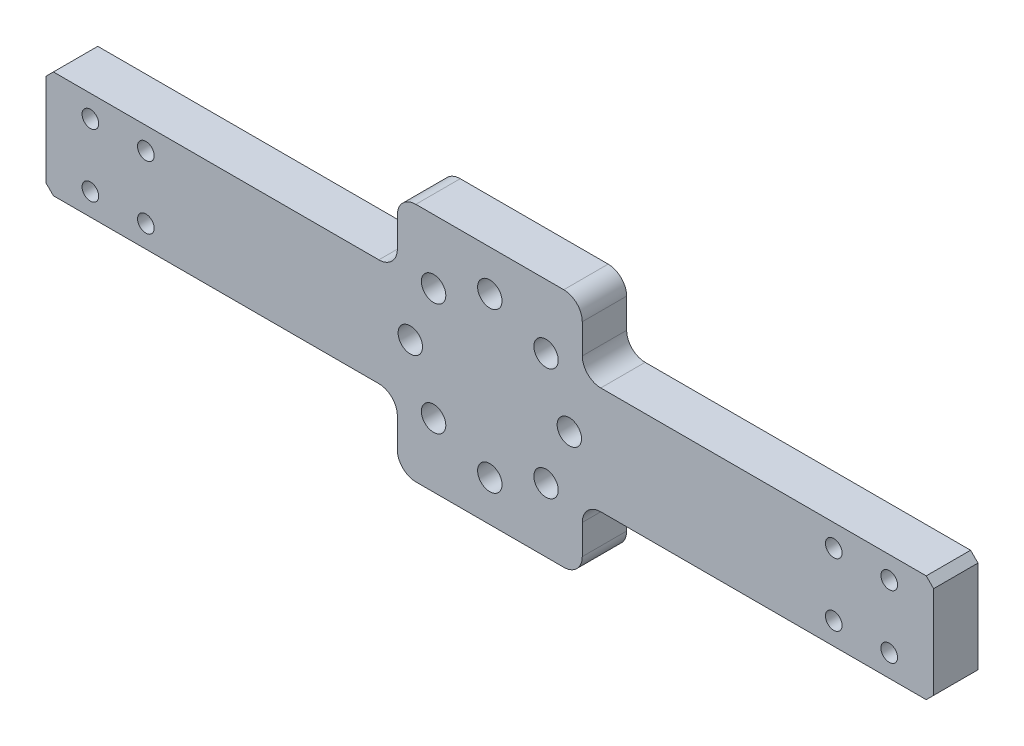
SolidWorks part; units mm, degrees
ref_plane "Front Plane" through (0, 0, 0) normal (0, 0, 1) x (1, 0, 0)
ref_plane "Top Plane" through (0, 0, 0) normal (0, 1, 0) x (1, 0, 0)
ref_plane "Right Plane" through (0, 0, 0) normal (1, 0, 0) x (0, 0, -1)
sketch "Sketch1" plane through (0, 0, 0) normal (0, 0, 1) x (1, 0, 0)
  line L1 (-120, 32.5) -> (120, 32.5)
  line L2 (-120, 32.5) -> (-120, -32.5)
  line L3 (-120, -32.5) -> (120, -32.5)
  line L4 (120, 32.5) -> (120, -32.5)
  line L5 (-120, 32.5) -> (120, -32.5) construction
  line L6 (-120, -32.5) -> (120, 32.5) construction
  point P0 (0, 0)
  dimension "D1" = 240
  dimension "D2" = 65
extrude "Boss-Extrude1" add sketch "Sketch1" along normal blind 12
sketch "Sketch2" plane through (0, 0, 12) normal (0, 0, 1) x (1, 0, 0)
  line L0 (0, 0) -> (0, 55.6312) construction
  line L2 (-120, 32.5) -> (-25, 32.5)
  line L4 (-120, 32.5) -> (-120, 14.5)
  line L5 (-120, 14.5) -> (-25, 14.5)
  line L6 (-25, 32.5) -> (-25, 14.5)
  line L7 (0, 0) -> (-139.8711, 0) construction
  line L8 (25, 32.5) -> (25, 14.5)
  line L9 (120, 14.5) -> (25, 14.5)
  line L10 (120, 32.5) -> (120, 14.5)
  line L11 (120, 32.5) -> (25, 32.5)
  line L12 (120, -32.5) -> (25, -32.5)
  line L13 (120, -32.5) -> (120, -14.5)
  line L14 (120, -14.5) -> (25, -14.5)
  line L15 (25, -32.5) -> (25, -14.5)
  line L16 (-25, -32.5) -> (-25, -14.5)
  line L17 (-120, -14.5) -> (-25, -14.5)
  line L18 (-120, -32.5) -> (-120, -14.5)
  line L19 (-120, -32.5) -> (-25, -32.5)
  dimension "D1" = 95
  dimension "D2" = 18
extrude "Cut-Extrude1" cut sketch "Sketch2" against normal through all both and the other way through all
fillet "Fillet1" radius 5 8 edges at (25, -32.5, 6) (-25, -32.5, 6) (25, 32.5, 6) (-25, 32.5, 6) (-25, -14.5, 6) (25, -14.5, 6) (25, 14.5, 6) (-25, 14.5, 6)
hole_wizard "Hole for socket head cap screw, type1" positions "Sketch4" profile "Sketch3" counterbore size "M6" standard "GB"
sketch "Sketch4" plane through (0, 0, 0) normal (0, 0, -1) x (-1, 0, 0)
  point P1 (15.2028, -15.2028)
  point P5 (0, -21.5)
  point P9 (-15.2028, -15.2028)
  point P13 (-21.5, 0)
  point P17 (-15.2028, 15.2028)
  point P21 (0, 21.5)
  point P25 (15.2028, 15.2028)
  point P29 (21.5, 0)
  dimension "D1" = 15.2028
  dimension "D2" = 15.2028
  dimension "D3" = 21.5
  dimension "D4" = 21.5
  dimension "D5" = 15.2028
  dimension "D6" = 15.2028
  dimension "D7" = 21.5
  dimension "D8" = 21.5
sketch "Sketch3" plane through (-15.2028, -15.2028, 0) normal (1, 0, 0) x (0, 1, 0)
  line L0 (0, 0) -> (0, 12)
  line L1 (0, 12) -> (3.3, 12)
  line L3 (3.3, 12) -> (3.3, 6.8)
  line L4 (3.3, 6.8) -> (5.5, 6.8)
  line L5 (5.5, 6.8) -> (5.5, 0)
  line L7 (5.5, 0) -> (0, 0)
  line L11 (0, -6.35) -> (0, 107.95) construction
  dimension "通孔孔直径" = 6.6
  dimension "通孔孔深度" = 12
  dimension "柱形沉头孔直径" = 11
  dimension "柱形沉头孔深度" = 6.8
hole_wizard "Ø4.5 (4.5) Diameter Hole1" positions "Sketch6" profile "Sketch5" hole size "Ø4.5" standard "GB"
sketch "Sketch6" plane through (0, 0, 12) normal (0, 0, 1) x (1, 0, 0)
  point P1 (-93, -8.5)
  point P5 (-108, -8.5)
  point P9 (-93, 8.5)
  point P13 (-108, 8.5)
  dimension "D1" = 15
  dimension "D2" = 93
  dimension "D3" = 8.5
  dimension "D4" = 8.5
sketch "Sketch5" plane through (-93, -8.5, 12) normal (1, 0, 0) x (0, -1, 0)
  line L0 (0, 0) -> (0, 12)
  line L1 (0, 12) -> (2.25, 12)
  line L2 (2.25, 12) -> (2.25, 0)
  line L5 (2.25, 0) -> (0, 0)
  line L11 (0, -6.35) -> (0, 107.95) construction
  dimension "通孔孔直径" = 4.5
  dimension "通孔孔深度" = 12
mirror "Mirror1" about plane through (0, 0, 0) normal (1, 0, 0) of "Ø4.5 (4.5) Diameter Hole1"
chamfer "Chamfer1" distance 2 angle 45 4 edges at (120, 14.5, 6) (120, -14.5, 6) (-120, -14.5, 6) (-120, 14.5, 6)
